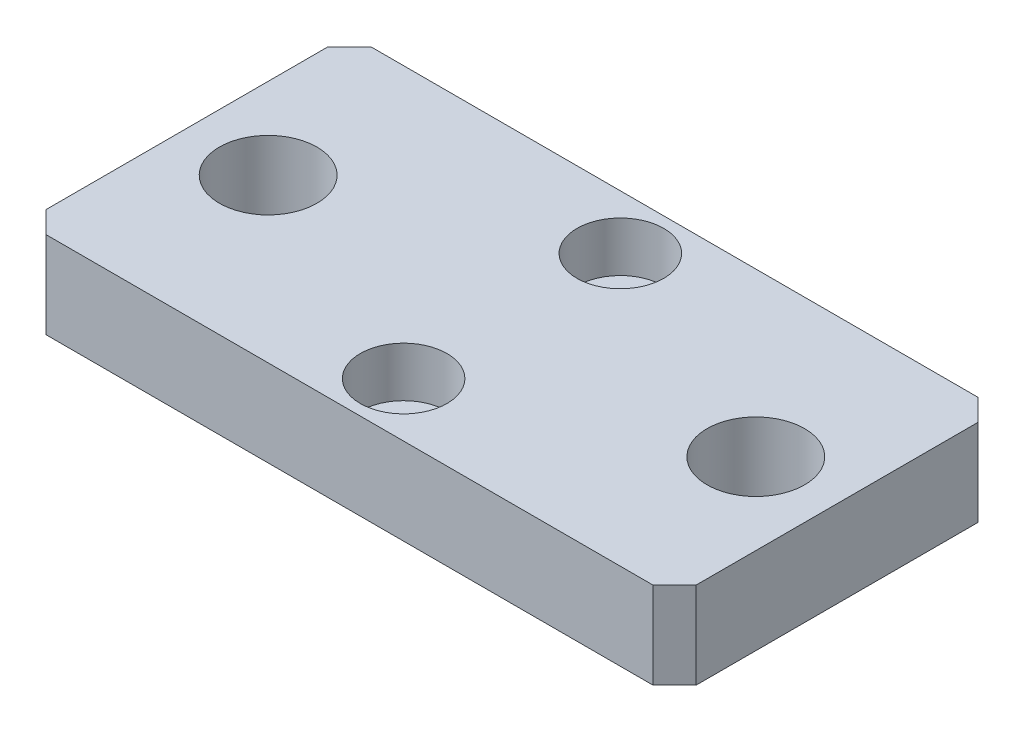
from build123d import *

# Parameters (mm, degrees)
SKETCH_1_W                = 60
SKETCH_1_H                = 30
EXTRUDE_1_DEPTH           = 4
CHAMFER_1_SIZE            = 2
HOLE_WIZARD_1_D           = 4.5
HOLE_WIZARD_1_CBORE_D     = 8
HOLE_WIZARD_1_CBORE_DEPTH = 4.6
M10X1_0_1_D               = 9


with BuildPart() as part:
    # 草图1 → 凸台-拉伸1 (new, symmetric)
    with BuildSketch(Plane(origin=(0, 0, 0), x_dir=(1, 0, 0), z_dir=(0, 1, 0))):
        Rectangle(SKETCH_1_W, SKETCH_1_H)
    extrude(amount=EXTRUDE_1_DEPTH, both=True)

    # 倒角1
    chamfer_1_edges = [part.edges().sort_by_distance(p)[0] for p in [
        (30, 0, 15),
        (-30, 0, 15),
        (-30, 0, -15),
        (30, 0, -15),
    ]]
    chamfer(chamfer_1_edges, length=CHAMFER_1_SIZE)

    # 打孔尺寸(%根据)内六角圆柱头螺钉的类型1 (through all)
    with Locations(Plane(origin=(0, 4, 0), x_dir=(1, 0, 0), z_dir=(0, 1, 0))):
        with Locations((0, -10), (0, 10)):
            CounterBoreHole(HOLE_WIZARD_1_D / 2, HOLE_WIZARD_1_CBORE_D / 2, HOLE_WIZARD_1_CBORE_DEPTH)

    # M10x1.0 螺纹孔1 (through all)
    with Locations(Plane(origin=(0, -4, 0), x_dir=(-1, 0, 0), z_dir=(0, -1, 0))):
        with Locations((-22.5, 0), (22.5, 0)):
            Hole(M10X1_0_1_D / 2)


solid = part.part
